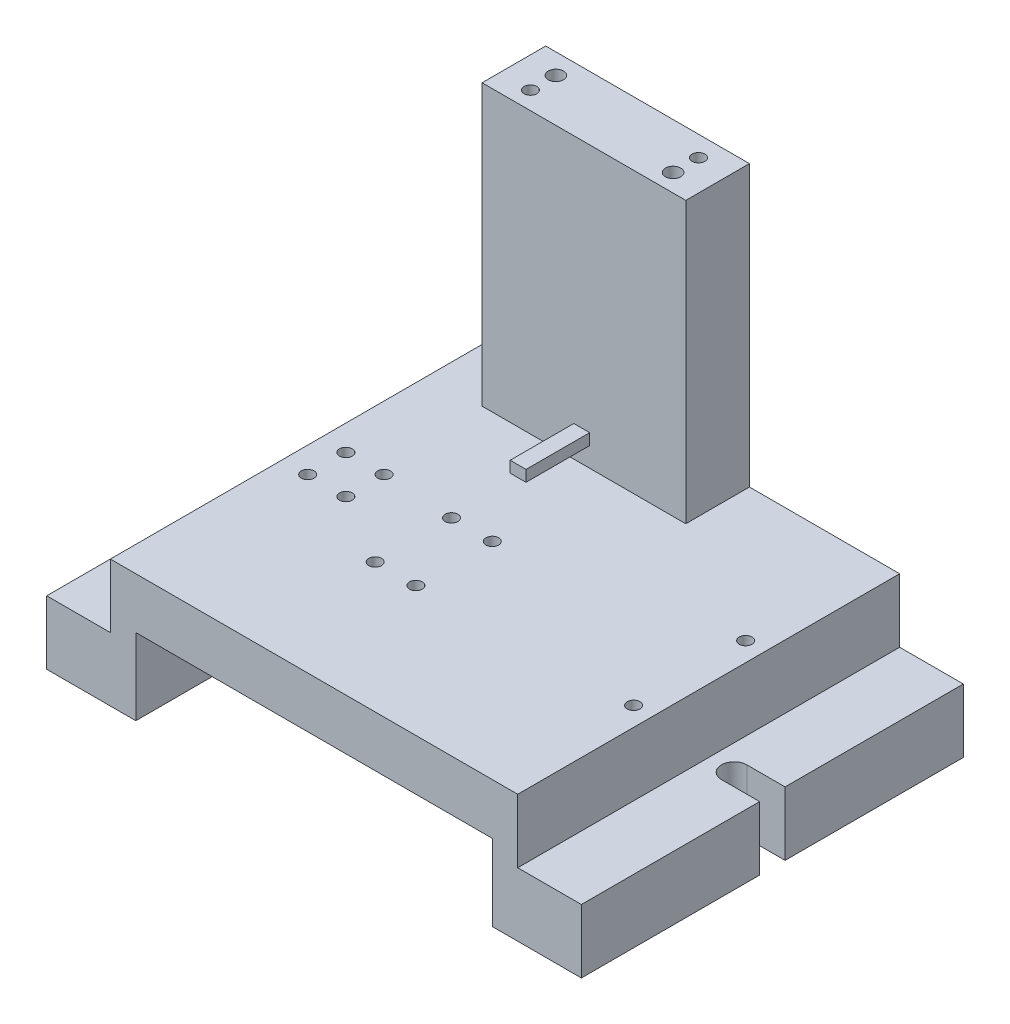
SolidWorks part; units mm, degrees
ref_plane "Front Plane" through (0, 0, 0) normal (0, 0, 1) x (1, 0, 0)
ref_plane "Top Plane" through (0, 0, 0) normal (0, 1, 0) x (1, 0, 0)
ref_plane "Right Plane" through (0, 0, 0) normal (1, 0, 0) x (0, 0, -1)
sketch "Sketch1" plane through (0, 0, 0) normal (0, 0, 1) x (1, 0, 0)
  line L0 (0, 0) -> (0, 25)
  line L1 (0, 25) -> (25, 25)
  line L2 (25, 25) -> (25, 50)
  line L3 (25, 50) -> (185, 50)
  line L4 (175, 30) -> (35, 30)
  line L5 (0, 0) -> (35, 0)
  line L6 (35, 0) -> (35, 30)
  line L7 (210, 0) -> (210, 25)
  line L8 (175, 0) -> (175, 30)
  line L9 (210, 0) -> (175, 0)
  line L10 (185, 25) -> (185, 50)
  line L11 (210, 25) -> (185, 25)
  dimension "D1" = 10
  dimension "D2" = 10
  dimension "D3" = 35
  dimension "D4" = 35
  dimension "D5" = 160
extrude "Boss-Extrude1" add sketch "Sketch1" along normal blind 150
sketch "Sketch9" plane through (0, 25, 0) normal (0, 1, 0) x (1, 0, 0)
  line L0 (210, -70) -> (210, -80)
  line L2 (15, -70) -> (0, -70)
  line L3 (15, -80) -> (0, -80)
  line L4 (0, -70) -> (0, -80)
  line L5 (185, 0) -> (25, 0) construction
  line L6 (105, 0) -> (105, -20.4747) construction
  line L7 (195, -80) -> (210, -80)
  line L8 (195, -70) -> (210, -70)
  arc A0 (15, -80) -> (15, -70) centre (15, -75) ccw
  arc A1 (195, -80) -> (195, -70) centre (195, -75) cw
extrude "Cut-Extrude1" cut sketch "Sketch9" against normal through all
hole_wizard "M6 Tapped Hole1" positions "Sketch11" profile "Sketch12" tap size "M6" standard "IS"
sketch "Sketch11" plane through (0, 50, 0) normal (0, 1, 0) x (1, 0, 0)
  point P0 (35, -82.5)
  point P2 (35, -67.5)
  point P4 (50, -67.5)
  point P6 (50, -82.5)
  point P8 (78, -69)
  point P10 (78, -99)
  point P12 (94, -69)
  point P14 (94, -99)
  point P16 (177.5, -97)
  point P18 (177.5, -53)
sketch "Sketch12" plane through (35, 50, 82.5) normal (1, 0, 0) x (0, 0, 1)
  line L0 (0, 0) -> (0, 16.5022)
  line L1 (0, 16.5022) -> (2.5, 15)
  line L2 (2.5, 15) -> (2.5, 0)
  line L5 (2.5, 0) -> (0, 0)
  line L10 (0, 16.5022) -> (-2.5, 15) construction
  line L11 (0, -6.35) -> (0, 107.95) construction
  dimension "螺纹孔钻头直径" = 5
  dimension "螺纹孔钻头深度" = 15
  dimension "导头角度" = 118
cosmetic thread "Cosmetic thread 1" parameters "D1"=12, "D2"=6
cosmetic thread "Cosmetic thread 2" parameters "D1"=12, "D2"=6
cosmetic thread "Cosmetic thread 3" parameters "D1"=12, "D2"=6
cosmetic thread "Cosmetic thread 4" parameters "D1"=12, "D2"=6
cosmetic thread "Cosmetic thread 5" parameters "D1"=12, "D2"=6
cosmetic thread "Cosmetic thread 6" parameters "D1"=12, "D2"=6
cosmetic thread "Cosmetic thread 7" parameters "D1"=12, "D2"=6
cosmetic thread "Cosmetic thread 8" parameters "D1"=12, "D2"=6
cosmetic thread "Cosmetic thread 9" parameters "D1"=12, "D2"=6
cosmetic thread "Cosmetic thread 10" parameters "D1"=12, "D2"=6
sketch "Sketch13" plane through (0, 50, 0) normal (0, 1, 0) x (1, 0, 0)
  line L0 (86, -45) -> (86, 0) construction
  line L1 (185, 0) -> (25, 0) construction
  line L2 (126, 0) -> (46, 0)
  line L3 (46, 0) -> (46, -25)
  line L4 (126, 0) -> (126, -25)
  line L5 (46, -25) -> (126, -25)
  dimension "D1" = 25
  dimension "D2" = 40
extrude "Boss-Extrude2" add sketch "Sketch13" along normal blind 110
hole_wizard "M6 Tapped Hole2" positions "Sketch16" profile "Sketch15" tap size "M6" standard "GB"
sketch "Sketch16" plane through (0, 160, 0) normal (0, 1, 0) x (1, 0, 0)
  point P0 (58, -18)
  point P3 (114, -8)
sketch "Sketch15" plane through (58, 160, 18) normal (1, 0, 0) x (0, 0, 1)
  line L0 (0, 0) -> (0, 16.5022)
  line L1 (0, 16.5022) -> (2.5, 15)
  line L2 (2.5, 15) -> (2.5, 0)
  line L5 (2.5, 0) -> (0, 0)
  line L10 (0, 16.5022) -> (-2.5, 15) construction
  line L11 (0, -6.35) -> (0, 107.95) construction
  dimension "螺纹孔钻头直径" = 5
  dimension "螺纹孔钻头深度" = 15
  dimension "导头角度" = 118
cosmetic thread "Cosmetic thread 11" parameters "D1"=12, "D2"=6
cosmetic thread "Cosmetic thread 12" parameters "D1"=12, "D2"=6
hole_wizard "Ø6.0mm dowel hole 1" positions "Sketch19" profile "Sketch18" hole size "Ø6.0" standard "GB"
sketch "Sketch19" plane through (0, 160, 0) normal (0, 1, 0) x (1, 0, 0)
  point P0 (58, -8)
  point P3 (114, -18)
sketch "Sketch18" plane through (58, 160, 8) normal (1, 0, 0) x (0, 0, 1)
  line L0 (0, 0) -> (0, 16.8026)
  line L1 (0, 16.8026) -> (3, 15)
  line L2 (3, 15) -> (3, 0)
  line L5 (3, 0) -> (0, 0)
  line L10 (0, 16.8026) -> (-3, 15) construction
  line L11 (0, -6.35) -> (0, 107.95) construction
  dimension "孔直径" = 6
  dimension "孔深度" = 15
  dimension "导头角度" = 118
sketch "Sketch20" plane through (0, 0, 25) normal (0, 0, 1) x (1, 0, 0)
  line L1 (82.0286, 62.1181) -> (88.2556, 62.1181)
  line L2 (82.0286, 62.1181) -> (82.0286, 57.7224)
  line L3 (82.0286, 57.7224) -> (88.2556, 57.7224)
  line L4 (88.2556, 62.1181) -> (88.2556, 57.7224)
  line L5 (82.0286, 62.1181) -> (88.2556, 57.7224) construction
  line L6 (82.0286, 57.7224) -> (88.2556, 62.1181) construction
  point P0 (85.1421, 59.9202)
extrude "Boss-Extrude3" add sketch "Sketch20" along normal blind 25
equation "\"A\"= \"代号代码\""
equation "\"B\"= \"名称代码\""
